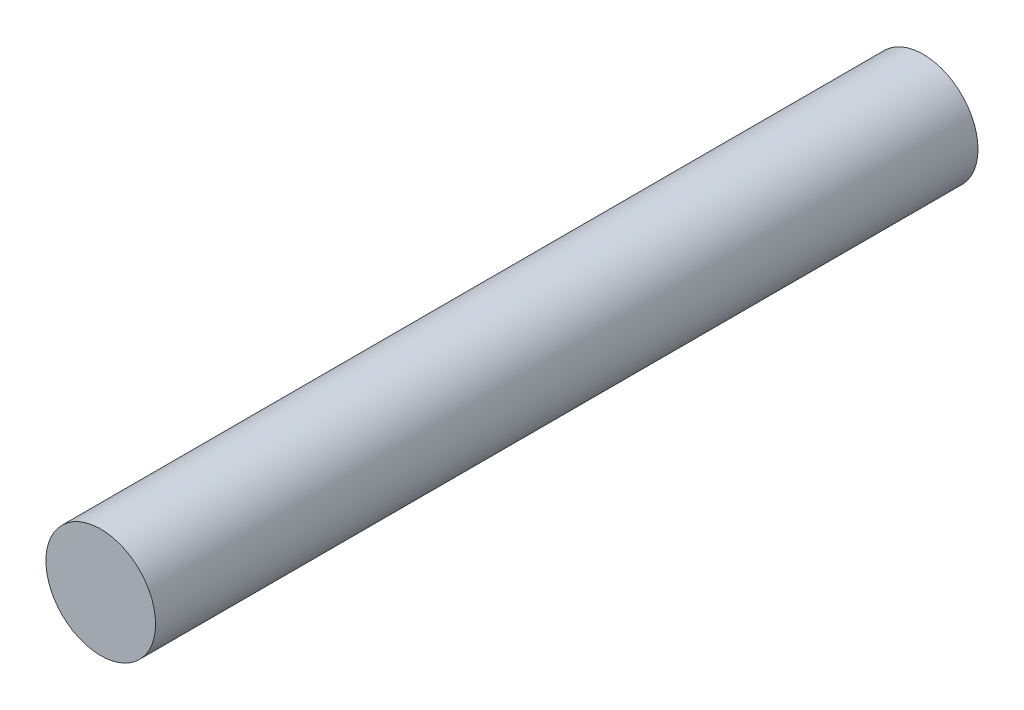
from build123d import *

# Parameters (mm, degrees)
SKETCH1_R           = 10
BOSS_EXTRUDE1_DEPTH = 150


with BuildPart() as part:
    # Sketch1 → Boss-Extrude1 (new body)
    with BuildSketch(Plane.XY):
        Circle(SKETCH1_R)
    extrude(amount=BOSS_EXTRUDE1_DEPTH)


solid = part.part
